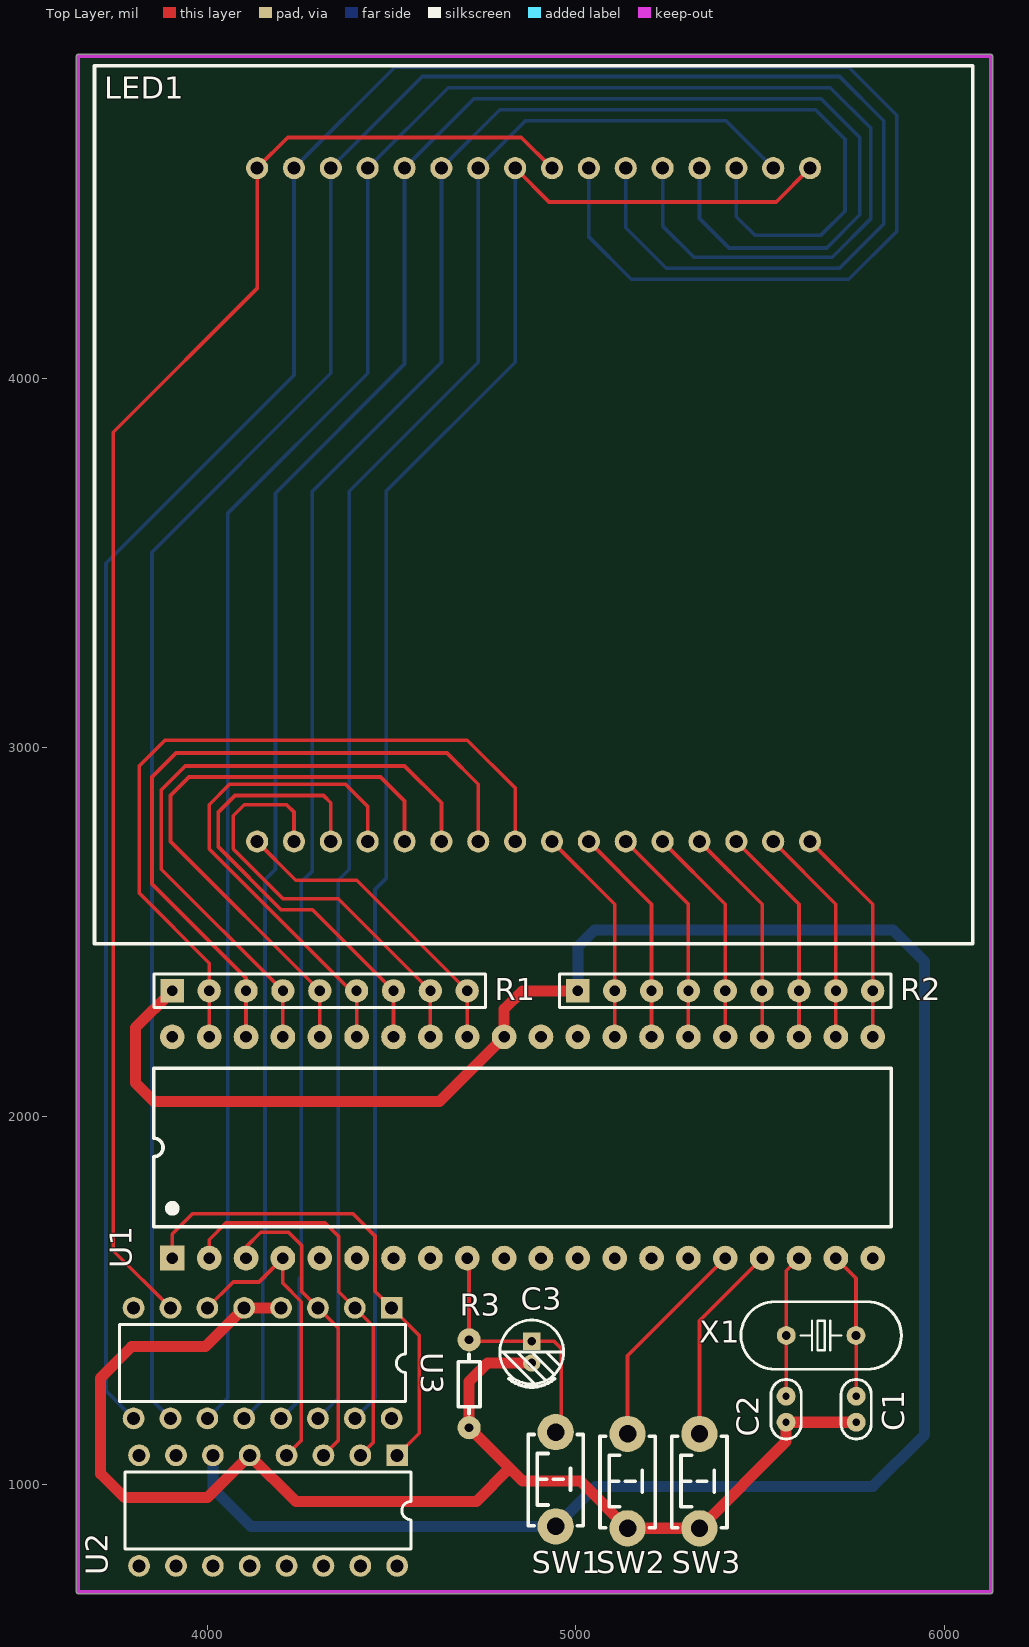
[diagram p0: Top Layer view]
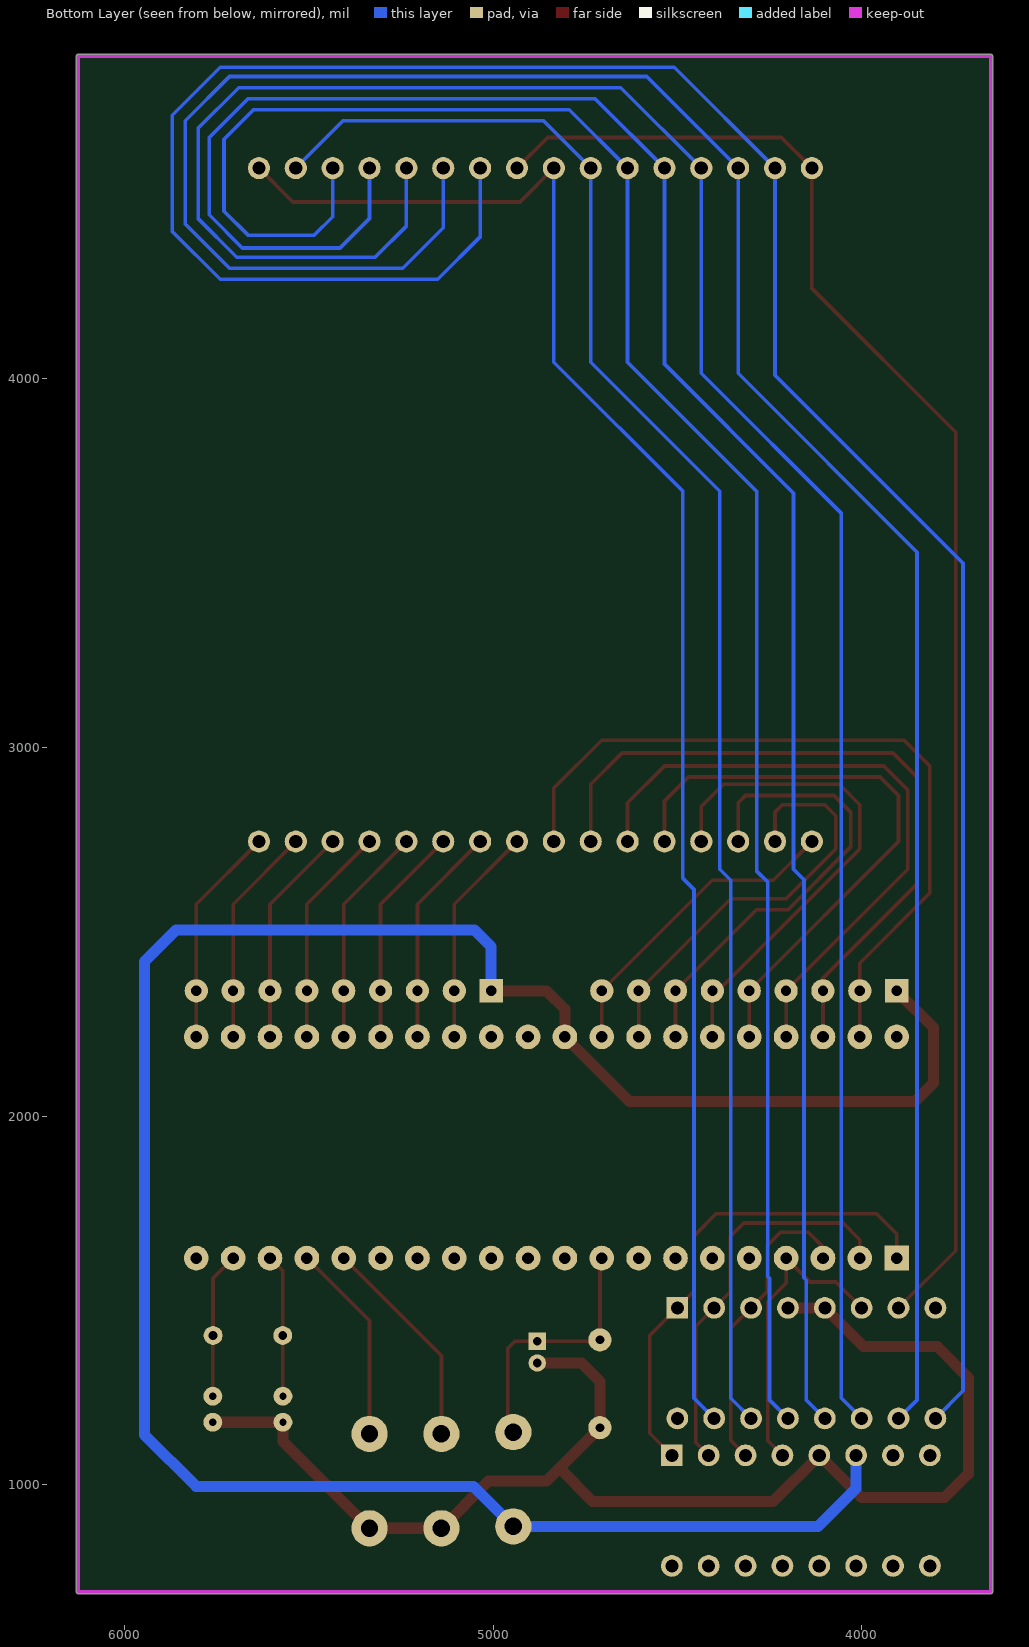
[diagram p1: Bottom Layer view, seen from below]
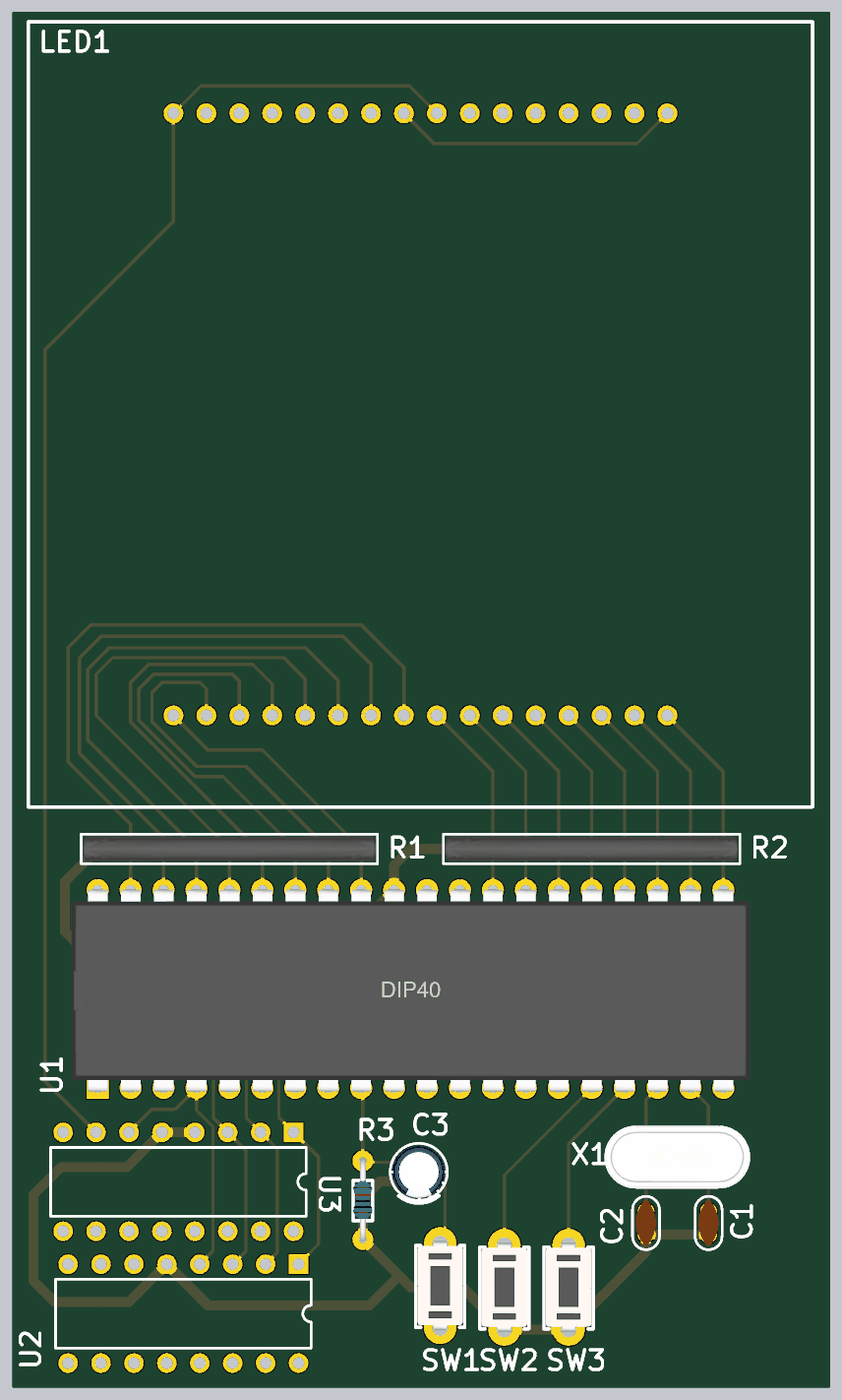
[diagram p2: 3D render of the assembled board from above, using the file's embedded part models]
# Altium PCB MISC80553.PcbDoc
Units mil, origin at the board's own origin, x right, y up, seen from the top; angles counter-clockwise.
Board outline 2485.03 x 4175.03 mil, 2 copper layers (Top Layer, Bottom Layer); 14 components, 47 nets, 138 pads, 0 vias.

## Layer stack, top to bottom (the 12.6 mil dielectric is the usual default, probably not edited)
Top Solder: solder mask 0.4, Solder Resist, Dk 3.5
Top Layer: signal copper 1.4
Dielectric 1: dielectric 12.6, FR-4, Dk 4.8
Bottom Layer: signal copper 1.4
Bottom Solder: solder mask 0.4, Solder Resist, Dk 3.5

## Board outline
3644.99,710 ccw(c3650,710) 3650,704.99 6125,704.99 ccw(c6125,710) 6130.02,710 6130.02,4875 ccw(c6125,4875) 6125,4880.02 3650,4880.02 ccw(c3650,4875) 3644.99,4875

## Design rules (kind name [scope] priority, off if disabled: settings)
Clearance [All] p1: gap=10
MinimumSolderMaskSliver [All] p1: minsoldermaskwidth=0
PolygonConnect [All] p1: connectstyle=Relief reliefconductorwidth=10 reliefentries=4 polygonreliefangle="90 Angle" airgapwidth=10
RoutingVias [All] p1: holewidth=28 width=50 viastyle="Through Hole" minholewidth=28 minwidth=50 maxholewidth=28 maxwidth=50
SilkToSilkClearance [All] p1: silktosilkclearance=0
SilkToSolderMaskClearance [IsPad] p1: minsilkscreentomaskgap=0 clearancetoexposedcopper=TRUE
SolderMaskExpansion [All] p1: expansion=4
Width [All] p1: maxlimit=30 minlimit=10 preferedwidth=10
27 further rules are at their usual default settings.

## Components (designator, comment, footprint, x,y, rotation, side; value= is the part's Value field where it differs from the comment)
C1 "30pF" "CC 1.8*3.6" 5760,1205 r90 top
C2 "30pF" "CC 1.8*3.6" 5570,1205 r90 top
C3 "10uF" "CAP 1.5*4*8" 4880,1360 r270 top
LED1 "RGB_Matrix_8x8" RGB_MATRIX_8X8 4885.01,3658.38 r0 top
R1 "561" "R SIP9-2.54" 4305,2340 r0 top
R2 "561" "R SIP9-2.54" 5405,2340 r0 top
R3 "10K" "RS 1/8W" 4710,1275 r90 top
SW1 "3x6x5" "TSW DIP-3*6*5" 4945,1015 r90 top
SW2 "3x6x5" "TSW DIP-3*6*5" 5140,1010 r90 top
SW3 "3x6x5" "TSW DIP-3*6*5" 5335,1010 r90 top
U1 "AT89C52" DIP40 4855,1915 r90 top
U2 "74HC138" 648-08 4165,930 r180 top
U3 "74HC138" 648-08 4150,1330 r180 top
X1 "12MHz" "OSC HC-49S" 5665,1405 r0 top

## Footprints (in the part's own frame and the unit in brackets; to place one, negate y for a bottom-side part, rotate by r counter-clockwise, add the part's x,y. Pads: shape width x height; smd on the part's side, far side on the other; paste and mask are expansions set on the pad)
648-08 [mm] "DIP; 16 Leads; Row Spacing 7.62 mm; Pitch 2.54 mm"
  rect 1.5x1.5 hole 0.9: 1(-8.89,-3.81)
  round 1.5 hole 0.9: 2(-6.35,-3.81) 3(-3.81,-3.81) 4(-1.27,-3.81) 5(1.27,-3.81) 6(3.81,-3.81) 7(6.35,-3.81) 8(8.89,-3.81) 9(8.89,3.81) 10(6.35,3.81) 11(3.81,3.81) 12(1.27,3.81) 13(-1.27,3.81) 14(-3.81,3.81) 15(-6.35,3.81) 16(-8.89,3.81)
  silkscreen extent -9.85,-2.65 9.85,2.65
"CAP 1.5*4*8" [mm] "脚距1.5mm直径4mm高度8mm"
  rect 1.2x1.2 hole 0.6: 1(-0.75,0)
  round 1.2 hole 0.6: 2(0.75,0)
  silkscreen extent -2.2,-2.2 2.41,2.2, body extent -2,-2 2.02,2, height 8.04
"CC 1.8*3.6" [mm] "脚距1.8mm直径3.6mm"
  round 1.3 hole 0.5: 1(-0.9,0) 2(0.9,0)
  silkscreen extent -2.05,-1.04 2.05,1.04, body extent -1.8,-0.8 1.8,0.8, height 3.6
DIP40 [mm]
  rect 1.7x1.7 hole 0.8: 1(-7.62,24.13)
  round 1.7 hole 0.8: 2(-7.62,21.59) 3(-7.62,19.05) 4(-7.62,16.51) 5(-7.62,13.97) 6(-7.62,11.43) 7(-7.62,8.89) 8(-7.62,6.35) 9(-7.62,3.81) 10(-7.62,1.27) 11(-7.62,-1.27) 12(-7.62,-3.81) 13(-7.62,-6.35) 14(-7.62,-8.89) 15(-7.62,-11.43) 16(-7.62,-13.97) 17(-7.62,-16.51) 18(-7.62,-19.05) 19(-7.62,-21.59) 20(-7.62,-24.13) 21(7.62,-24.13) 22(7.62,-21.59) 23(7.62,-19.05) 24(7.62,-16.51) 25(7.62,-13.97) 26(7.62,-11.43) 27(7.62,-8.89) 28(7.62,-6.35) 29(7.62,-3.81) 30(7.62,-1.27) 31(7.62,1.27) 32(7.62,3.81) 33(7.62,6.35) 34(7.62,8.89) 35(7.62,11.43) 36(7.62,13.97) 37(7.62,16.51) 38(7.62,19.05) 39(7.62,21.59) 40(7.62,24.13)
  silkscreen extent -5.46,-25.4 5.46,25.4, body extent -7.91,-26.19 7.65,26.16, height 4.7
"OSC HC-49S" [mm]
  round 1.3 hole 0.6: 1(-2.4,0) 2(2.4,0)
  silkscreen extent -5.52,-2.32 5.52,2.33, body extent -5.52,-2.32 5.53,2.33, height 4.13
"R SIP9-2.54" [mm] "22.6mm*5mm*2.2mm(长*宽*厚)"
  rect 1.6x1.6 hole 0.7: 1(-10.16,0)
  round 1.6 hole 0.7: 2(-7.62,0) 3(-5.08,0) 4(-2.54,0) 5(0,0) 6(2.54,0) 7(5.08,0) 8(7.62,0) 9(10.16,0)
  silkscreen extent -11.43,-1.14 11.43,1.14, body extent -11.31,-0.96 11.31,0.96, height 5.2
RGB_MATRIX_8X8 [mil]
  round 60 hole 36 paste+4 mask+4: 1(-750.01,-913.38) 2(-650.01,-913.38) 3(-550.01,-913.38) 4(-450.01,-913.38) 5(-350.01,-913.38) 6(-250.01,-913.38) 7(-150.01,-913.38) 8(-50.01,-913.38) 9(49.99,-913.38) 10(149.99,-913.38) 11(249.99,-913.38) 12(349.99,-913.38) 13(449.99,-913.38) 14(549.99,-913.38) 15(649.99,-913.38) 16(749.99,-913.38) 17(749.99,913.39) 18(649.99,913.39) 19(549.99,913.39) 20(449.99,913.39) 21(349.99,913.39) 22(249.99,913.39) 23(149.99,913.39) 24(49.99,913.39) 25(-50.01,913.39) 26(-150.01,913.39) 27(-250.01,913.39) 28(-350.01,913.39) 29(-450.01,913.39) 30(-550.01,913.39) 31(-650.01,913.39) 32(-750.01,913.39)
  silkscreen extent -1191,-1191 1191,1191
"RS 1/8W" [mm] "直插色环电阻，脚距6mm，直径1.5mm"
  round 1.6 hole 0.6: 1(-3.048,0) 2(3,0)
  silkscreen extent -2.1,-0.75 2,0.75, body extent -3.22,-0.76 3.23,0.76, height 1.52
"TSW DIP-3*6*5" [mm] "3*6*5mm"
  round 2.5 hole 1.2: 1(3.25,0) 2(-3.25,0)
  silkscreen extent -3.21,-1.9 3.09,1.9, body extent -3.91,-1.75 3.91,1.75, height 5.01

## Part data
C1 C2: library part C, "Non-polar SMD capacitor"
C3: library part C-CAP, "THT electrolytic capacitor"
R1 R2: library part "R SIP9", "Single in-line resistor array"
R3: library part R, "SMD resistor"
SW1 SW2 SW3: library part "TSW 3x6", "3x6 tact switch"
U2 U3: library part Component_1
X1: library part XTAL-2P, "2-pin passive crystal"

## Nets (pads, with @x,y where several pads share a name; then routed paths per layer and width w, separated by ;. In a path a pad name is that pad's centre, name@x,y a point inside that pad or via, vN(x,y) a via of type N, cw(c..) or ccw(c..) an arc to the next point about the centre after c; other vN are vias at no path point)
GND: C1.1 C2.1 C3.2 R3.1 SW2.2 SW3.2 U2.5 U3.4 U3.5 | length 3731.1
  Top Layer w30: U3.4 U3.5 3995,1375 3795,1375 3710,1290 3710,1030 3775,965 4000,965 U2.5 4240,955 4730,955 4820,1045 ; C3.2 4760.47,1330.47 4710,1280 R3.1 4820,1045 ; C1.1 C2.1 5570,1117.05 SW3.2 SW2.2 5012.05,1010 4855,1010 4820,1045
NetC1_2: C1.2 U1.19 X1.2 | length 397.3
  Top Layer w10: U1.19 5759.49,1560.51 X1.2 5760,1404.49 C1.2
NetC2_2: C2.2 U1.18 X1.1 | length 389.1
  Top Layer w10: C2.2 5570,1404.49 X1.1 5570.51,1580.51 U1.18
NetC3_1: C3.1 R3.2 SW1.1 U1.9 | length 716.8
  Top Layer w10: U1.9 4710,1610 R3.2 4713.58,1389.53 C3.1 4940.47,1389.53 4960,1370 4960,1157.95 SW1.1
NetSW2_1: SW2.1 U1.16 | length 586.8
  Top Layer w10: SW2.1 5140,1350 U1.16
NetSW3_1: SW3.1 U1.17 | length 547.5
  Top Layer w10: SW3.1 5335,1445 U1.17
P1.0: U1.1 U2.1 U3.1 | length 1332.2
  Top Layer w10: U1.1 3905,1680 3960,1735 4395,1735 4455,1675 4455,1525 U3.1 4575,1405 4575,1140 U2.1
P1.1: U1.2 U2.2 U3.2 | length 1082
  Top Layer w10: U1.2 4005,1665 4050,1710 4320,1710 4356.54,1673.46 4356.54,1523.46 U3.2 4450,1430 4450,1115 U2.2
P1.2: U1.3 U2.3 U3.3 | length 839.1
  Top Layer w10: U1.3 4105,1645 4145,1685 4220,1685 4256.54,1648.46 4256.54,1523.46 U3.3 4355,1425 4355,1120 U2.3
P1.3: U1.4 U2.4 U3.6 | length 833.2
  Top Layer w10: U3.6 4070,1550 4140,1550 U1.4 4205,1546.72 4255,1496.72 4255,1120 U2.4
P1.4: U1.5
P1.5: U1.6
P1.6: U1.7
P1.7: U1.8
VCC: R1.1 R2.1 SW1.2 U1.31 U2.6 | length 6244.5
  Top Layer w30: R1.1 3805,2240 3805,2090 3855,2040 4630,2040 U1.31 4805,2290 4855,2340 R2.1
  Bottom Layer w30: U2.6 4015,990 4117.95,887.05 SW1.2 5052.95,995 5805,995 5945,1135 5945,2420 5860,2505 5050,2505 5005,2460 R2.1
X0: U2.15
X1: U2.14
X2: U2.13
X3: U2.12
X4: U2.11
X5: U2.10
X6: U2.9
X7: U2.7
X8: LED1.17 LED1.25 U3.15 | length 4448
  Top Layer w10: LED1.25 4926.77,4480 5543.23,4480 LED1.17
  Bottom Layer w10: U3.15 4455,1235 4455,2615 4485,2645 4485,3695 4835,4045 LED1.25
X9: LED1.18 LED1.26 U3.14 | length 4478.2
  Bottom Layer w10: U3.14 4355,1235 4355,2640 4385,2670 4385,3695 4735,4045 LED1.26 4863.23,4700 5406.77,4700 LED1.18
X10: LED1.19 LED1.27 U3.13 | length 5435
  Bottom Layer w10: U3.13 4250,1230 4250,1560 4255,1565 4255,2635 4285,2665 4285,3695 4635,4045 LED1.27 4793.23,4730 5650,4730 5730,4650 5730,4455 5665,4390 5485,4390 5435,4440 LED1.19
X11: LED1.20 LED1.28 U3.12 | length 5780.6
  Bottom Layer w10: U3.12 4150,1230 4150,1555 4156.54,1561.54 4156.54,2641.54 4185,2670 4185,3690 4535,4040 LED1.28 4723.23,4760 5665,4760 5770,4655 5770,4445 5680,4355 5415,4355 5335,4435 LED1.20
X12: LED1.21 LED1.29 U3.11 | length 6118.4
  Bottom Layer w10: U3.11 4055,1235 4055,3635 4435,4015 LED1.29 4653.23,4790 5690,4790 5800,4680 5800,4435 5695,4330 5320,4330 5235,4415 LED1.21
X13: LED1.22 LED1.30 U3.10 | length 6502.9
  Bottom Layer w10: U3.10 3850,1230 3850,3530 4335,4015 LED1.30 4583.23,4820 5715,4820 5835,4700 5835,4420 5715,4300 5245,4300 5135,4410 LED1.22
X14: LED1.23 LED1.31 U3.9 | length 6874.4
  Bottom Layer w10: U3.9 3725,1255 3725,3500 4235,4010 LED1.31 4508.23,4845 5740,4845 5870,4715 5870,4400 5740,4270 5150,4270 5035,4385 LED1.23
X15: LED1.24 LED1.32 U3.7 | length 4186.5
  Top Layer w10: U3.7 3745,1635 3745,3855 4135,4245 LED1.32 4218.23,4655 4851.77,4655 LED1.24
Y0: LED1.1 R1.9 U1.32 | length 862.8
  Top Layer w10: LED1.1 4240,2640 4405,2640 R1.9 U1.32
Y1: LED1.2 R1.8 U1.33 | length 1175.2
  Top Layer w10: LED1.2 4235,2825 4215,2845 4100,2845 4070,2815 4070,2725 4205,2590 4355,2590 R1.8 U1.33
Y2: LED1.3 R1.7 U1.34 | length 1293.5
  Top Layer w10: LED1.3 4335,2850 4315,2870 4075,2870 4030,2825 4030,2730 4200,2560 4285,2560 R1.7 U1.34
Y3: LED1.4 R1.6 U1.35 | length 1377.1
  Top Layer w10: U1.35 R1.6 4390,2340 4005,2725 4005,2845 4060,2900 4375,2900 4435,2840 LED1.4
Y4: LED1.5 R1.5 U1.36 | length 1615.4
  Top Layer w10: U1.36 R1.5 3900,2745 3900,2870 3950,2920 4470,2920 4535,2855 LED1.5
Y5: LED1.6 R1.4 U1.37 | length 1740
  Top Layer w10: U1.37 R1.4 3875,2670 3875,2885 3940,2950 4535,2950 4635,2850 LED1.6
Y6: LED1.7 R1.3 U1.38 | length 1912.8
  Top Layer w10: U1.38 R1.3 4105,2375 3850,2630 3850,2920 3915,2985 4650,2985 4735,2900 LED1.7
Y7: LED1.8 R1.2 U1.39 | length 2061.5
  Top Layer w10: U1.39 R1.2 4005,2415 3815,2605 3815,2950 3885,3020 4705,3020 4835,2890 LED1.8
Y8: LED1.9 R2.2 U1.28 | length 600.4
  Top Layer w10: LED1.9 5105,2575 R2.2 U1.28
Y9: LED1.10 R2.3 U1.27 | length 600.4
  Top Layer w10: LED1.10 5205,2575 R2.3 U1.27
Y10: LED1.11 R2.4 U1.26 | length 600.4
  Top Layer w10: LED1.11 5305,2575 R2.4 U1.26
Y11: LED1.12 R2.5 U1.25 | length 600.4
  Top Layer w10: LED1.12 5405,2575 R2.5 U1.25
Y12: LED1.13 R2.6 U1.24 | length 600.4
  Top Layer w10: LED1.13 5505,2575 R2.6 U1.24
Y13: LED1.14 R2.7 U1.23 | length 600.4
  Top Layer w10: LED1.14 5605,2575 R2.7 U1.23
Y14: LED1.15 R2.8 U1.22 | length 600.4
  Top Layer w10: LED1.15 5705,2575 R2.8 U1.22
Y15: LED1.16 R2.9 U1.21 | length 600.4
  Top Layer w10: LED1.16 5805,2575 R2.9 U1.21
pads on no net: U1.10 U1.11 U1.12 U1.13 U1.14 U1.15 U1.20 U1.29 U1.30 U1.40 U2.8 U2.16 U3.8 U3.16

## Keep-outs
Keep-Out Layer:
  lines w10: 5980,710 6125,710 6125,4875 3900,4875 3650,4875 3650,710 6005,710